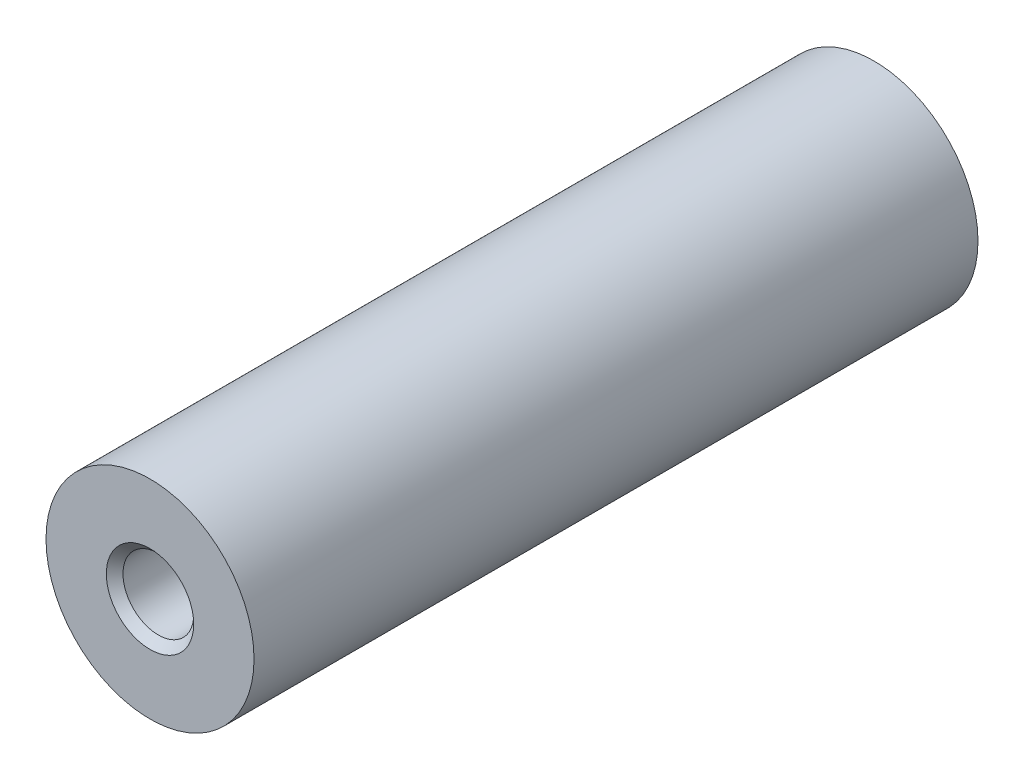
from build123d import *

# Parameters (mm, degrees)
SKETCH1_R           = 12.5
BOSS_EXTRUDE1_DEPTH = 87
SKETCH2_R           = 4.25
CUT_EXTRUDE1_DEPTH  = 25
CHAMFER1_SIZE       = 1


with BuildPart() as part:
    # Sketch1 → Boss-Extrude1 (new body)
    with BuildSketch(Plane.XY):
        Circle(SKETCH1_R)
    extrude(amount=BOSS_EXTRUDE1_DEPTH)

    # Sketch2 → Cut-Extrude1 (cut)
    with BuildSketch(Plane.XY.offset(87)):
        Circle(SKETCH2_R)
    extrude(amount=-CUT_EXTRUDE1_DEPTH, mode=Mode.SUBTRACT)

    # Chamfer1
    chamfer1_edges = [part.edges().sort_by_distance(p)[0] for p in [
        (-4.25, 0, 87),
    ]]
    chamfer(chamfer1_edges, length=CHAMFER1_SIZE)


solid = part.part
